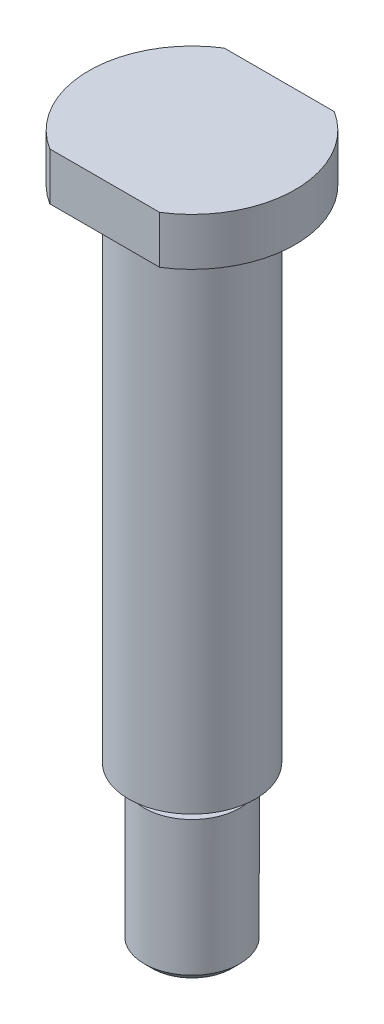
SolidWorks part; units mm, degrees
material "45#"
ref_plane "前基準面" through (0, 0, 0) normal (0, 0, 1) x (1, 0, 0)
ref_plane "上基準面" through (0, 0, 0) normal (0, 1, 0) x (1, 0, 0)
ref_plane "右基準面" through (0, 0, 0) normal (1, 0, 0) x (0, 0, -1)
sketch "草图1" plane through (0, 0, 0) normal (0, 1, 0) x (1, 0, 0)
  circle A0 centre (0, 0) radius 4
  dimension "D1" = 8
extrude "凸台-拉伸1" add sketch "草图1" along normal blind 31.5
sketch "草图2" plane through (0, 0, 0) normal (0, -1, 0) x (1, 0, 0)
  circle A0 centre (0, 0) radius 3
  dimension "D1" = 6
extrude "凸台-拉伸2" add sketch "草图2" along normal blind 10
cosmetic thread "装饰螺纹线1" parameters "D2"=4.917
sketch "草图3" plane through (0, 31.5, 0) normal (0, 1, 0) x (1, 0, 0)
  circle A0 centre (0, 0) radius 6.5
  dimension "D1" = 13
extrude "凸台-拉伸3" add sketch "草图3" along normal blind 3
sketch "草图4" plane through (0, 34.5, 0) normal (0, 1, 0) x (1, 0, 0)
  line L1 (-6.5, -5.5) -> (6.5, -5.5)
  line L2 (-6.5, -5.5) -> (-6.5, 5.5)
  line L3 (-6.5, 5.5) -> (6.5, 5.5)
  line L4 (6.5, -5.5) -> (6.5, 5.5)
  line L5 (-6.5, -5.5) -> (6.5, 5.5) construction
  line L6 (-6.5, 5.5) -> (6.5, -5.5) construction
  circle A0 centre (0, 0) radius 6.5 construction
  point P0 (0, 0)
  point P8 (0, 6.5)
  dimension "D1" = 1
extrude "切除-拉伸1" cut sketch "草图4" against normal through all flip side to cut
chamfer "倒角1" distance 0.5 angle 45 1 edges at (0, -10, -3)
sketch "草图5" plane through (0, 0, 0) normal (0, 0, 1) x (1, 0, 0)
  line L0 (0, 0) -> (0, -6.5367) construction
  line L1 (-3, 0) -> (-2.5, 0)
  line L2 (-3, 0) -> (-3, -1)
  line L3 (-3, -1) -> (-2.5, -1)
  line L4 (-2.5, 0) -> (-2.5, -1)
  dimension "D1" = 1
  dimension "D2" = 0.5
revolve "切除-旋转1" cut sketch "草图5" angle 360 about L0
